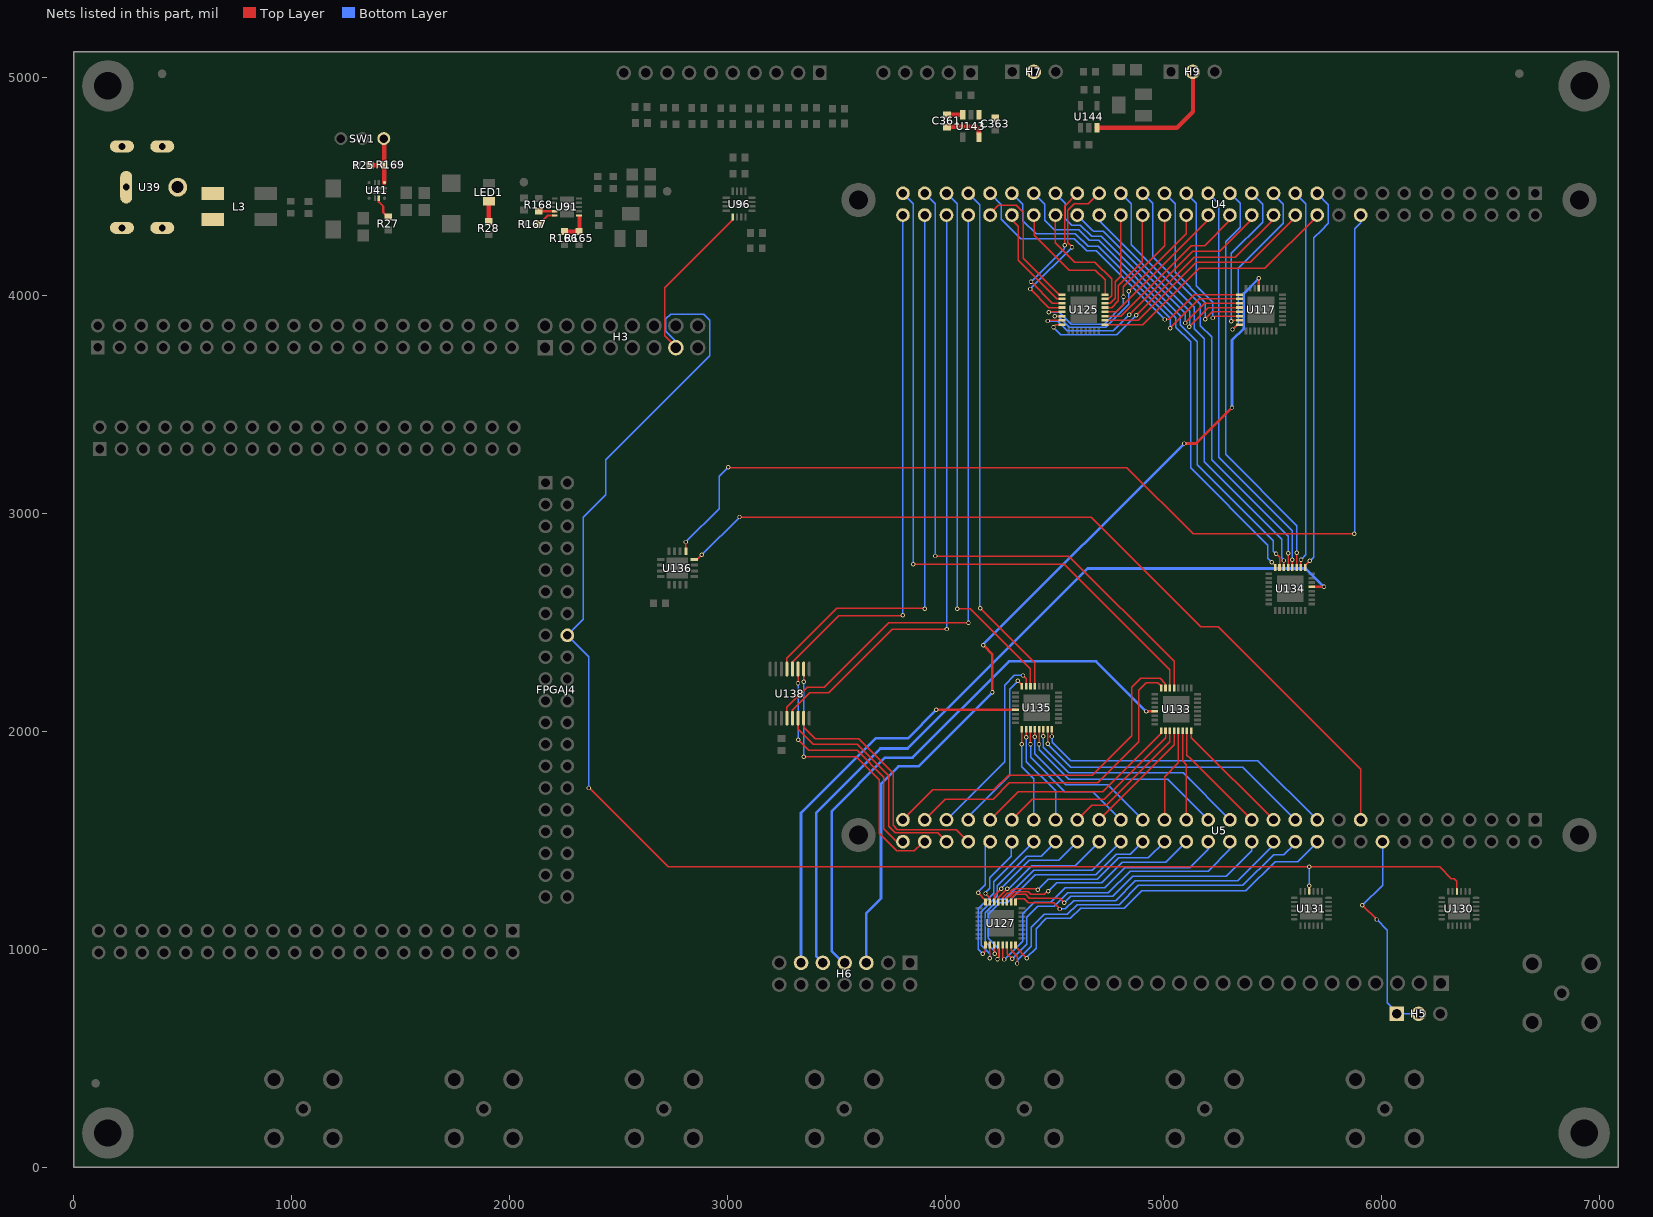
[diagram p0: the nets of this part, all layers, seen from the top]
# Altium PCB MISC82799.PcbDoc (part 4 of 5)
Units mil, origin at the board's own origin, x right, y up, seen from the top; angles counter-clockwise.
Board outline 7086.61 x 5118.11 mil, 4 copper layers (Top Layer, GND, POWER, Bottom Layer); 95 components, 232 nets, 857 pads, 1291 vias.

## Via types
v1: diameter 20, hole 12, Top Layer to Bottom Layer, 1291 vias

## Nets (pads, with @x,y where several pads share a name; then routed paths per layer and width w, separated by ;. In a path a pad name is that pad's centre, name@x,y a point inside that pad or via, vN(x,y) a via of type N, cw(c..) or ccw(c..) an arc to the next point about the centre after c; other vN are vias at no path point) (continued)
NetC361_1: C361.1 U143.3 | length 65.4
  Top Layer w20: C361.1@4006.33,4827.69 U143.3@4071.69,4827.69
NetC361_2: C361.2 U143.5 | length 171.3
  Top Layer w20: C361.2@4006.33,4772.57 4138.43,4772.57 4152,4759 U143.5@4152,4739
NetC363_2: C363.2 H7.2 U143.1
NetH9_2: H9.2 U144.3 | length 654.8
  Top Layer w20: U144.3@4693.96,4767.82 5060.82,4767.82 5135,4842 H9.2@5135,5025
NetL3_1: L3.1 U39.1
NetL3_2: L3.2 U39.2 U39.3
NetLED1_2: LED1.2 R28.2 | length 84.6
  Top Layer w20: R28.2@1905,4347 LED1.2@1905,4431.65
NetR25_2: R25.2 R169.1 SW1.3 U41.1 | length 243.7
  Top Layer w20: R25.2@1360.66,4597 R169.1@1423,4597 ; U41.1@1425.34,4516 R169.1@1425.34,4598 SW1.3@1425.34,4697.34
NetR27_1: R27.1 U41.9 | length 95.3
  Top Layer w10: U41.9@1399.86,4445.37 1399.86,4429.14 1421,4408 1421,4380 R27.1@1436,4365
NetR165_1: R165.1 R166.2 U91.6 | length 137
  Top Layer w20: R166.2@2252,4291.66 2320.66,4291.66 2320.66,4360
NetR167_2: R167.2 U91.5 | length 73.7
  Top Layer w10: R167.2@2146,4336 2175.63,4365.63 U91.5@2207.43,4365.63
NetR168_1: R168.1 U91.4 | length 72.1
  Top Layer w10: R168.1@2135.31,4385.31 U91.4@2207.43,4385.31
PSUB: H5.1 H5.2 U5.16 | length 960.6
  Top Layer w6: v1(5912,1202) v1(5977,1137)
  Bottom Layer w6: v1(5912,1202) 6004.35,1294.35 U5.16@6004.35,1493.8 ; v1(5977,1137) 6026,1088 6026,755 H5.1@6063,718 ; H5.1@6070,704 H5.2@6154,704
S_D_11: U4.26 U125.8 | length 1304.3
  Top Layer w6: v1@4496,3855 4506.1,3865.1 U125.8@4534.58,3865.1 ; v1(4874,3908) 5140,4174 5329,4174 5504.35,4349.35 U4.26@5504.35,4367.81
  Bottom Layer w6: v1(4495,3853) 4529,3819 4785,3819 v1(4874,3908)
S_D_12: U4.28 U125.7 | length 1249.2
  Top Layer w6: v1@4469.78,3884.78 U125.7@4534.58,3884.78 ; v1(4843,3911) 5133,4201 5257,4201 5404.35,4348.35 U4.28@5404.35,4367.81
  Bottom Layer w6: v1(4469,3882) 4515,3882 4559,3838 4770,3838 v1(4843,3911)
S_D_13: U5.28 U127.2 | length 1285.4
  Top Layer w6: U127.2@4301.22,1217.43 4301.22,1233.22 4320,1252 4368,1252 4385,1235 4524,1235 v1(4545,1214)
  Bottom Layer w6: v1@4543,1212 v1(4545,1214) 4575,1244 4767,1244 4859,1336 5288,1336 5404.35,1452.35 U5.28@5404.35,1493.8
S_D_14: U5.26 U127.1 | length 1389.9
  Top Layer w6: U127.1@4320.9,1217.43 4320.9,1225.9 4326,1231 4362,1231 4380,1213 ; 4424,1213 4380,1213 ; v1(4524,1185) 4496,1213 4380,1213
  Bottom Layer w6: v1@4528,1185 4550,1185 4588,1223 4780,1223 4871,1314 5340,1314 U5.26@5504,1478 ; U5.26@5504.35,1478 U5.26@5504.35,1493.8
S_D_21: U4.34 U125.6 | length 946.3
  Top Layer w6: v1(4501,3904) 4502,3905 U125.6@4526,3905 ; v1(4840,4019) 5104.35,4283.35 U4.34@5104.35,4367.81
  Bottom Layer w6: v1(4501,3904) 4517,3904 4567,3854 4734,3854 4840,3960 v1(4840,4019)
S_D_22: U4.36 U125.5 | length 953.5
  Top Layer w6: v1@4473.16,3924.15 U125.5@4534.58,3924.15 ; v1(4816,3993) 4816,4039 5004.35,4227.35 U4.36@5004.35,4367.81
  Bottom Layer w6: v1(4473,3923) 4522,3923 4577,3868 4728,3868 4816,3956 v1(4816,3993)
S_D_23: U5.36 U127.4 | length 892.5
  Top Layer w6: U127.4@4261.84,1217.43 4261.84,1229 U127.4@4261.84,1232.85 ; U127.4@4262,1229 4262,1236 4283.97,1257.97 4292,1257.97 ; 4292.06,1258 4304.53,1270.47 ; 4307.53,1273.47 4304.53,1270.47 ; 4380,1278 4363,1278 ; v1@4419,1274 4415,1278 4363,1278 ; 4304.53,1270.47 4312.06,1278 4363,1278
  Bottom Layer w6: v1(4423,1273) 4472,1322 4696,1322 4794,1420 4930.55,1420 U5.36@5004.35,1493.8
S_D_24: U5.34 U127.3 | length 954.2
  Top Layer w6: U127.3@4281.52,1217.43 4281.52,1234.52 4291,1244 4295,1244 4297,1246 4315.03,1264 4321,1264 ; 4320,1264 4321,1264 ; v1@4467,1267 4452,1252 4391,1252 4379,1264 4321,1264
  Bottom Layer w6: v1(4471,1267) 4510,1306 4717,1306 4810,1399 5009.55,1399 U5.34@5104.35,1493.8
S_D_31: U4.41 U125.4 | length 804.5
  Top Layer w6: v1(4388,4029) 4389,4029 4474.16,3943.85 U125.4@4534.58,3943.85 ; v1@4578,4224 4561,4241 4561,4390 4591,4420 4655,4420 U4.41@4696,4461 ; v1(4580,4221) v1@4580,4224 ; U4.41@4696.77,4460.23 U4.41@4704.35,4467.81
  Bottom Layer w6: v1(4388,4029) v1(4580,4221)
S_D_32: U4.43 U125.3 | length 672.3
  Top Layer w6: v1(4392,4062) 4490.48,3963.52 U125.3@4534.58,3963.52 ; v1@4546,4230 4546,4409.46 U4.43@4604.35,4467.81
  Bottom Layer w6: v1(4392,4062) 4544,4214 v1@4544,4226
  other v1: 4546,4229
S_D_33: U5.44 U127.6 | length 508.1
  Top Layer w6: U127.6@4222.48,1217.43 4222.48,1246.48 v1@4252,1276
  Bottom Layer w6: v1@4256,1279 4385,1408 4518.55,1408 U5.44@4604.35,1493.8
  other v1: 4256,1278
S_D_34: U5.42 U127.5 | length 590.9
  Top Layer w6: U127.5@4242.16,1217.43 4242.16,1236.15 4279,1273 4281.03,1275 v1@4283,1275 ; v1(4283,1278) 4283,1277 4285,1275 v1@4284,1274
  Bottom Layer w6: v1@4284,1273 4287,1276 v1@4287,1278 ; v1@4290,1278 4396,1384 4594.55,1384 U5.42@4704.35,1493.8
S_D_41: U4.50 U125.2 | length 472.6
  Top Layer w6: U4.50@4303,4346 4333,4316 4333,4161 4510.78,3983.22 U125.2@4534.58,3983.22
S_D_42: U4.52 U125.1 | length 630.5
  Top Layer w6: U4.52@4210,4381 4241,4412 4324,4412 4356,4380 4356,4169 4522.1,4002.9 U125.1@4534.58,4002.9
S_D_43: U5.52 U127.8 | length 306.2
  Top Layer w6: v1(4150,1259) 4183.1,1225.9 U127.8@4183.1,1217.43
  Bottom Layer w6: v1@4151,1265 4181,1295 4181,1470.45 U5.52@4204.35,1493.8
S_D_44: U5.50 U127.7 | length 311.1
  Top Layer w6: v1(4183,1256) 4202.78,1236.22 U127.7@4202.78,1217.43
  Bottom Layer w6: v1@4182,1259 4202,1279 4202,1328 4301,1427 U5.50@4301,1474
S_D_51: U4.58 U138.13 | length 2578.5
  Top Layer w6: U138.13@3272.21,2285.82 3272.21,2334.21 3502,2564 v1@3901,2564
  Bottom Layer w6: v1(3904.35,2561.65) U4.58@3904.35,4367.81
S_D_52: U4.60 U138.12 | length 2460.9
  Top Layer w6: U138.12@3297.8,2285.82 3297.8,2315.8 3511,2529 v1@3805,2529
  Bottom Layer w6: v1(3804.35,2532.35) U4.60@3804.35,4367.81
S_D_53: U5.60 U138.11 | length 1152.7
  Top Layer w6: v1@3323.39,2227.61 U138.11@3323.39,2285.82 ; v1(3324,1961) 3373,1912 3594,1912 3717,1789 3717,1764 ; 3717,1787 3717,1764 ; U5.60@3804.35,1493.8 3777.2,1493.8 3717,1554 3717,1764
  Bottom Layer w6: v1(3323,2220) 3324,2220 v1(3324,1961)
S_D_54: U5.58 U138.10 | length 1321.7
  Top Layer w6: v1(3349,1883) 3590,1883 3695,1778 3695,1724 ; v1(3349,2227) U138.10@3349,2262 ; 3695,1773 3695,1724 ; U5.58@3890,1485 3857,1452 3775,1452 3695,1532 3695,1724 ; U5.58@3892.78,1482.22 U5.58@3904.35,1493.8
  Bottom Layer w6: v1(3349,1883) v1(3349,2227)
S_G_11: U4.22 U125.17 | length 1172.9
  Top Layer w6: U125.17@4731.42,3865.1 4905.1,3865.1 5164,4124 5465,4124 5697,4356 U4.22@5697,4360
S_G_12: U4.24 U125.18 | length 1069.3
  Top Layer w6: U125.18@4731.42,3884.78 4884.78,3884.78 5151,4151 5397,4151 5601,4355 U4.24@5601,4360
S_G_13: U5.24 U127.23 | length 1666.2
  Top Layer w6: U127.23@4301.22,1020.57 4301.22,994.78 4328,968 v1(4328,935)
  Bottom Layer w6: v1@4330,936 4330,952 4392,1014 4392,1101 4452,1161 4559,1161 4603,1205 4797,1205 4885,1293 5364,1293 5505,1434 5552,1434 U5.24@5603,1485 ; U5.24@5604.35,1485 U5.24@5604.35,1493.8
S_G_14: U5.22 U127.24 | length 1687.5
  Top Layer w6: U127.24@4320.9,1020.57 4320.9,1011.1 v1(4373,959)
  Bottom Layer w6: v1@4373,963 4416,1006 4416,1095 4463,1142 4573,1142 4619,1188 4819,1188 4899,1268 5378,1268 5512,1402 5616,1402 U5.22@5694,1480 ; U5.22@5692.28,1481.72 U5.22@5704.35,1493.8
S_G_21: U4.30 U125.19 | length 773.4
  Top Layer w6: U125.19@4737,3905 4804,3905 5127,4228 5189,4228 5304.35,4343.35 U4.30@5304.35,4367.81
S_G_22: U4.32 U125.20 | length 660
  Top Layer w6: U125.20@4731.42,3924.15 4782.16,3924.15 U4.32@5213,4355
S_G_23: U5.32 U127.21 | length 1318.7
  Top Layer w6: U127.21@4261.84,1020.57 4261.84,961.15 v1@4266,957
  Bottom Layer w6: v1(4269,953) 4353,1037 4353,1163 4407,1217 4483,1217 4548,1282 4730,1282 4822,1374 5119.35,1374 5204,1458.65 U5.32@5204,1479 ; U5.32@5204.35,1479 U5.32@5204.35,1493.8
S_G_24: U5.30 U127.22 | length 1388.5
  Top Layer w6: U127.22@4282,1013 4282,980 v1(4306,956)
  Bottom Layer w6: v1(4306,956) 4373,1023 4373,1148 4423,1198 4499,1198 4560,1259 4635,1259 ; 4628,1259 4635,1259 ; U5.30@5304.35,1493.8 5304.35,1459.35 5204,1359 4847,1359 4747,1259 4635,1259
S_G_31: U4.38 U125.21 | length 496.6
  Top Layer w6: U125.21@4731.42,3943.85 4762.84,3943.85 4793,3974 4793,4044 4903,4154 U4.38@4903,4351
S_G_32: U4.40 U125.22 | length 427.7
  Top Layer w6: U125.22@4731.42,3963.52 4755.52,3963.52 4778,3986 4778,4061 4804,4087 U4.40@4804,4347
S_G_33: U5.40 U127.19 | length 1001
  Top Layer w6: v1@4222.48,984.52 U127.19@4222.48,1020.57
  Bottom Layer w6: v1(4225,979) 4225,991 4181,1035 4181,1167 4244,1230 4252,1230 4256,1230 4272,1230 4404,1362 4672.55,1362 U5.40@4804.35,1493.8
S_G_34: U5.38 U127.20 | length 1132.6
  Top Layer w6: v1@4240,958 4245,963 4245,991 4242.16,993.85 U127.20@4242.16,1020.57
  Bottom Layer w6: 4246,962 4246,1000 4195,1051 4195,1148 4195,1151 4195,1160 4248,1213 4282,1213 4412,1343 4689,1343 4782,1436 4846.55,1436 U5.38@4904.35,1493.8
  other v1: 4238,954
S_G_41: U4.46 U125.23 | length 566
  Top Layer w6: U4.46@4504,4366 4504,4240 4592,4152 4685,4152 4762,4075 4762,3998 4747.22,3983.22 U125.23@4731.42,3983.22
S_G_42: U4.48 U125.24 | length 560.2
  Top Layer w6: U4.48@4407,4354 4407,4276 4567,4116 4686,4116 4731.42,4070.58 U125.24@4731.42,4002.9 ; U4.48@4408,4354 U4.48@4408,4359
S_G_43: U5.48 U127.17 | length 673.9
  Top Layer w6: v1(4171,979) 4183.1,991.1 U127.17@4183.1,1020.57
  Bottom Layer w6: v1@4170,980 4150,1000 4150,1187 4221,1258 4221,1310 U5.48@4389,1478 ; U5.48@4388.78,1478.22 U5.48@4404.35,1493.8
S_G_44: U5.46 U127.18 | length 792.2
  Top Layer w6: v1(4202.78,959.78) U127.18@4202.78,1020.57
  Bottom Layer w6: v1(4202.78,959.78) 4202.78,979.22 4164,1018 4164,1173 4237,1246 4237,1292 4373,1428 4438.55,1428 U5.46@4504.35,1493.8 ; v1@4203,961 v1@4203,963
S_G_51: U4.54 U138.4 | length 2925.7
  Top Layer w6: U138.4@3272.21,2060.18 3272.21,2109.21 3365,2202 3444,2202 3740,2498 v1(4105,2498)
  Bottom Layer w6: v1@4104.35,2498.35 4104.35,2816 ; 4104.35,2802.65 4104.35,2816 ; U4.54@4104.35,4367.81 4104.35,2816
S_G_52: U4.56 U138.5 | length 2809.8
  Top Layer w6: U138.5@3297.8,2060.18 3297.8,2096.8 3378,2177 3464,2177 3756,2469 v1(4005,2469)
  Bottom Layer w6: v1@4004.35,2469.35 4004.35,2788 ; 4004.35,2774.65 4004.35,2788 ; U4.56@4004.35,4367.81 4004.35,2788
S_G_53: U5.56 U138.6 | length 1081.1
  Top Layer w6: U138.6@3323.39,2060.18 3323.39,2009.61 3393,1940 3595,1940 3739,1796 3739,1564 3768.71,1534.29 3963.85,1534.29 U5.56@4004.35,1493.8
S_G_54: U5.54 U138.7 | length 1154.7
  Top Layer w6: U138.7@3348.98,2060.18 3348.98,2019.02 3402,1966 3601,1966 3759,1808 3759,1568 3779,1548 4050.14,1548 U5.54@4104.35,1493.8
S_N_LEFT: U4.18 U136.9 | length 4937
  Top Layer w6: U136.9@2808.39,2825.77 v1(2808.39,2868.39) ; v1@3004,3214 3008,3210 4832,3210 5135,2907 v1(5875,2907)
  Bottom Layer w6: v1(2808.39,2868.39) 2961,3021 2961,3169 v1(3003,3211) ; v1(5875,2907) 5876,2908 5876,4305 5904.35,4333.35 U4.18@5904.35,4367.81
S_N_RIGHT: U5.17 U136.8 | length 3852.7
  Top Layer w6: U136.8@2846.77,2787.39 2859.39,2787.39 v1(2882,2810) ; v1@3053,2985 v1(3055,2983) 3056,2982 4669,2982 5171,2480 5250,2480 5904.35,1825.65 U5.17@5904.35,1593.8
  Bottom Layer w6: v1(2882,2810) v1(3055,2983)
S_S_11: U4.25 U117.8 | length 757.9
  Top Layer w6: v1(5316,3843) 5338.1,3865.1 U117.8@5348.58,3865.1
  Bottom Layer w6: v1(5316,3843) 5342,3869 5342,4123 5550,4331 5550,4406 5550,4417 U4.25@5518,4449
S_S_12: U4.27 U117.7 | length 698.4
  Top Layer w6: v1@5316.78,3884.78 U117.7@5348.58,3884.78
  Bottom Layer w6: v1(5311,3881) 5311,4193 5454,4336 5454,4418.16 U4.27@5404.35,4467.81
S_S_13: U5.27 U133.7 | length 531.9
  Top Layer w6: U133.7@5107,1997 5107,1891.14 5121.57,1876.57 U5.27@5404.35,1593.8 ; U133.7@5107.22,1997 U133.7@5107.22,2002.57
S_S_14: U5.25 U133.8 | length 565.2
  Top Layer w6: U133.8@5126.9,2002.57 5126.9,1971.1 5138,1960 ; 5138.07,1960.07 U5.25@5504.35,1593.8
S_S_21: U4.33 U117.6 | length 743.3
  Top Layer w6: v1(5225,3896) v1@5229,3896 ; v1@5228,3895 v1@5229,3896 ; U117.6@5348.58,3904.48 5237.48,3904.48 v1@5229,3896
  Bottom Layer w6: U4.33@5104.35,4467.81 5150,4422.16 5150,4043 5225,3968 v1@5225,3903
S_S_22: U4.35 U117.5 | length 821.4
  Top Layer w6: v1(5192,3890) 5192,3892 5224.16,3924.15 U117.5@5348.58,3924.15
  Bottom Layer w6: U4.35@5004.35,4467.81 5053,4419.16 5053,4105 5192,3966 v1@5192,3896
S_S_23: U5.35 U133.5 | length 429.6
  Top Layer w6: U5.35@5004.35,1593.8 5004.35,1791.35 5068,1855 U133.5@5068,1997
S_S_24: U5.33 U133.6 | length 415.7
  Top Layer w6: U133.6@5087.52,2002.57 5087.52,1864.48 5104.35,1847.65 U5.33@5104.35,1593.8
S_S_31: U4.42 U117.4 | length 962.7
  Top Layer w6: v1@5116,3854 5205.84,3943.85 U117.4@5348.58,3943.85
  Bottom Layer w6: U4.42@4704.35,4367.81 4704.35,4342.65 5121,3926 5121,3858 v1(5118,3855) ; v1@5115,3852 v1(5118,3855) ; v1@5118,3853 v1(5118,3855)
S_S_32: U4.44 U117.3 | length 1013.9
  Top Layer w6: v1@5098,3873 5099,3873 5189.52,3963.52 U117.3@5348.58,3963.52
  Bottom Layer w6: U4.44@4604.35,4367.81 4673.08,4299.08 ; 4673,4299 4679,4293 4724,4293 5099,3918 v1(5099,3873.16)
S_S_33: U5.43 U133.3 | length 622.6
  Top Layer w6: U5.43@4604.35,1593.8 4670.55,1660 4737,1660 5028,1951 U133.3@5028,2002
S_S_34: U5.41 U133.4 | length 550.6
  Top Layer w6: U5.41@4704.35,1593.8 5048,1937.45 U133.4@5048,2002
S_S_41: U4.49 U117.2 | length 1433.9
  Top Layer w6: v1@5024,3848 5028,3848 5163.22,3983.22 U117.2@5348.58,3983.22
  Bottom Layer w6: U4.49@4304.35,4467.81 4355,4417.16 4355,4343 4415,4283 4596,4283 4655,4224 4701,4224 5030,3895 v1(5030,3848)
S_S_42: U4.51 U117.1 | length 1465.5
  Top Layer w6: v1@5011,3889 5027,3889 5140.9,4002.9 U117.1@5348.58,4002.9
  Bottom Layer w6: U4.51@4204.35,4467.81 4256,4416.16 4256,4349 4345,4260 4591,4260 4647,4204 4691,4204 v1(5006,3889)
S_S_43: U5.51 U133.1 | length 953.6
  Top Layer w6: U5.51@4204.35,1593.8 4333.55,1723 4720,1723 4989,1992 U133.1@4989,1996
S_S_44: U5.49 U133.2 | length 891.5
  Top Layer w6: U5.49@4304.35,1593.8 4398.55,1688 4727,1688 5009,1970 U133.2@5009,2001
S_S_51: U4.57 U133.21 | length 3104.1
  Top Layer w6: v1(3953,2804) 4566,2804 5048.16,2321.85 U133.21@5048.16,2199.43
  Bottom Layer w6: U4.57@3904.35,4467.81 3953,4419.16 v1(3953,2804) v1@3955,2802
S_S_52: U4.59 U133.22 | length 3177.8
  Top Layer w6: v1(3852,2766) 4544,2766 5028.48,2281.52 U133.22@5028.48,2199.43
  Bottom Layer w6: U4.59@3804.35,4467.81 3852,4420.16 v1@3852,2769
S_S_53: U5.59 U133.23 | length 1627.2
  Top Layer w6: U5.59@3809,1600 3941,1732 4222,1732 4289,1799 4674,1799 4855,1980 4855,2203 4896,2244 4984,2244 5008.78,2219.22 U133.23@5008.78,2199.43
S_S_54: U5.57 U133.24 | length 1485.7
  Top Layer w6: U5.57@3904.35,1593.8 3999.55,1689 4219,1689 4293,1763 4699,1763 4887,1951 4887,2188 4921,2222 4974,2222 U133.24@4986,2210
S_W_11: U4.21 U134.1 | length 1784.9
  Top Layer w6: U134.1@5649.9,2751.43 5649.9,2761.9 v1(5670,2782)
  Bottom Layer w6: v1@5672,2782 5689,2799 5689,3031 ; 5689,3027 5689,3031 ; U4.21@5704.35,4467.81 5756,4416.16 5756,4330 5723,4297 5689,4263 5689,3031
S_W_12: U4.23 U134.2 | length 1744.4
  Top Layer w6: U134.2@5630.22,2751.43 v1(5630.22,2786.78)
  Bottom Layer w6: U4.23@5604.35,4467.81 5653,4419.16 5653,2810 v1@5631,2788
S_W_13: U5.23 U135.7 | length 1342.7
  Top Layer w6: v1(4468.22,1942.22) U135.7@4468.22,2009.57
  Bottom Layer w6: v1@4472,1939 4575,1836 5362.14,1836 U5.23@5604.35,1593.8
S_W_14: U5.21 U135.8 | length 1419.4
  Top Layer w6: v1(4487.9,1976.1) U135.8@4487.9,2009.57
  Bottom Layer w6: v1@4489,1973 4489,1950 4574,1865 4616,1865 5433.14,1865 U5.21@5704.35,1593.8
S_W_21: U4.29 U134.3 | length 1894
  Top Layer w6: U134.3@5610.52,2751.43 v1(5610.52,2818.52)
  Bottom Layer w6: U4.29@5304.35,4467.81 5351,4421.16 5351,4312 5285,4246 5285,3271 5612,2944 v1@5612,2823
S_W_22: U4.31 U134.4 | length 1872.4
  Top Layer w6: U134.4@5590.84,2751.43 v1(5590.84,2786.85)
  Bottom Layer w6: U4.31@5204.35,4467.81 5253,4419.16 5253,3257 5591,2919 v1@5591,2791
S_W_23: U5.31 U135.5 | length 1001.8
  Top Layer w6: v1(4428.84,1940.15) U135.5@4428.84,2009.57
  Bottom Layer w6: v1@4429,1939 4429,1915 4564,1780 5018.14,1780 U5.31@5204.35,1593.8
S_W_24: U5.29 U135.6 | length 1080.5
  Top Layer w6: v1(4448.52,1977.52) U135.6@4448.52,2009.57
  Bottom Layer w6: 4449,1958.52 4449,1952 ; v1@4449,1975 4449,1952 ; U5.29@5304.35,1593.8 5089.14,1809 4566,1809 4449,1926 4449,1952
S_W_31: U4.37 U134.5 | length 1986.8
  Top Layer w6: U134.5@5571.16,2751.43 v1(5571.16,2816.85)
  Bottom Layer w6: U4.37@4904.35,4467.81 4950,4422.16 4950,4177 5169,3958 5169,3860 5220,3809 5220,3246 5572,2894 v1@5572,2823
S_W_32: U4.39 U134.6 | length 2024.5
  Top Layer w6: U134.6@5551.48,2751.43 v1(5551.48,2783.48)
  Bottom Layer w6: U4.39@4804.35,4467.81 4852,4420.16 4852,4232 5140,3944 5140,3847 5186,3801 5186,3237 5542,2881 5542,2795 v1@5552,2785
S_W_33: U5.39 U135.3 | length 667.5
  Top Layer w6: v1(4389.48,1940.52) U135.3@4389.48,2009.57
  Bottom Layer w6: 4390,1921.52 4390,1916 ; v1@4390,1940 4390,1916 ; U5.39@4804.35,1593.8 4675.14,1723 4547,1723 4390,1880 4390,1916
S_W_34: U5.37 U135.4 | length 741.9
  Top Layer w6: v1(4409.16,1975.15) U135.4@4409.16,2009.57
  Bottom Layer w6: 4409,1955 4409,1941 ; v1@4409,1969 4409,1941 ; U5.37@4904.35,1593.8 4744.14,1754 4551,1754 4409,1896 4409,1941
S_W_41: U4.45 U134.7 | length 2196.2
  Top Layer w6: v1(5516,2814) 5531.78,2798.22 U134.7@5531.78,2751.43
  Bottom Layer w6: U4.45@4504.35,4467.81 4550,4422.16 4550,4350 4578,4322 4618,4322 4670,4270 4713,4270 5076,3907 5076,3864 5154,3786 5154,3223 5495.5,2881.5 ; 5499.5,2877.5 5495.5,2881.5 ; v1(5516,2814) 5503,2827 5503,2874 5495.5,2881.5
S_W_42: U4.47 U134.8 | length 2266
  Top Layer w6: v1(5496,2776) 5512.1,2759.9 U134.8@5512.1,2751.43
  Bottom Layer w6: U4.47@4404.35,4467.81 4454,4418.16 4454,4345 4499,4300 4611,4300 4659,4252 4702,4252 5057,3897 5057,3854 5124,3787 5124,3208 5478,2854 5478,2794 v1(5496,2776)
S_W_43: U5.47 U135.1 | length 436.2
  Top Layer w6: v1(4350.1,1940.1) U135.1@4350.1,2009.57
  Bottom Layer w6: v1@4350,1938 4350,1837 4404.35,1782.65 U5.47@4404.35,1593.8
S_W_44: U5.45 U135.2 | length 473.4
  Top Layer w6: v1(4369.78,1972.78) U135.2@4369.78,2009.57
  Bottom Layer w6: 4370,1953.78 4370,1947 ; v1@4370,1968 4370,1947 ; U5.45@4504.35,1593.8 4504.35,1726.65 4370,1861 4370,1947
S_W_51: U4.53 U135.21 | length 2383.8
  Top Layer w6: v1(4159,2564) 4409.16,2313.85 U135.21@4409.16,2206.43
  Bottom Layer w6: U4.53@4104.35,4467.81 4157,4415.16 v1@4157,2567
S_W_52: U4.55 U135.22 | length 2458.6
  Top Layer w6: v1(4053,2562) 4114,2562 4389.48,2286.52 U135.22@4389.48,2206.43
  Bottom Layer w6: U4.55@4004.35,4467.81 4053,4419.16 4053,2799 ; v1@4053,2564 4053,2799 ; 4053,2795 4053,2799
S_W_53: U5.55 U135.23 | length 886
  Top Layer w6: v1(4355,2256) 4369.78,2241.22 U135.23@4369.78,2206.43
  Bottom Layer w6: U5.55@4004.35,1593.8 4271,1860.45 4271,2211 4316,2256 v1(4355,2256)
S_W_54: U5.53 U135.24 | length 762.6
  Top Layer w6: v1(4331,2232) 4350.1,2212.9 U135.24@4350.1,2206.43
  Bottom Layer w6: U5.53@4104.35,1593.8 4104.35,1608.35 4294,1798 4294,2192 v1@4331,2229
SCLK: FPGAJ4.16 H3.13 U96.13 U130.22 U131.22 | length 7907.7
  Top Layer w6: v1@2365,1740 2727,1378 5269,1378 ; H3.13@2756,3770 2712,3814 2712,4034 3023.48,4345.48 U96.13@3023.48,4358.94 ; 5246,1378 5269,1378 ; v1@5664,1378 v1@5668.2,1378 ; U131.22@5668.2,1265.74 v1(5668.2,1291.8) ; U130.22@6345.2,1265.74 6345.2,1289 ; 6345.2,1292 6345.2,1289 ; 5269,1378 v1@5668.2,1378 ; v1@5668.2,1378 6266,1378 6320,1324 6333,1324 6345.2,1311.8 6345.2,1289
  Bottom Layer w6: 2328,2503 2325,2500 ; v1(2363,1740) 2363,2342 FPGAJ4.16@2265,2440 2325,2500 ; H3.13@2760,3771 2760,3792 2717,3835 2717,3892 2739,3914 2891,3914 2919,3886 2919,3723 2442,3246 2442,3085 2338,2981 2338,2513 2325,2500 ; H3.13@2763,3740 H3.13@2763,3741 ; v1(5668.2,1291.8) v1(5668.2,1379.2)
SOURCE_LEFT: H6.5 U117.29 | length 4052.5
  Top Layer w12: v1(4173,2395) 4215,2353 v1(4215,2179) ; v1(5095,3320) 5149,3320 v1(5314,3485) ; U117.29@5437.16,4032.42 v1(5437.16,4078.16)
  Bottom Layer w12: H6.5@3637,938 3637,1166 3704,1233 3704,1759 3784,1839 3875,1839 v1(4215,2179) ; v1@4170,2395 v1(5095,3320) ; v1(5314,3485) 5314,3794 5368,3848 5368,4009 v1(5437.16,4078.16)
SOURCE_RIGHT: H6.7 U133.29 | length 2579.3
  Top Layer w12: v1(4920.16,2091.15) U133.29@4959.58,2091.15
  Bottom Layer w12: H6.7@3531,938 3478,991 3478,1634 3723,1879 3849,1879 4291,2321 4690.31,2321 v1(4920.16,2091.15)
WELL_LEFT: H6.9 U134.29 | length 3585.5
  Top Layer w12: U134.29@5679.42,2662.85 v1(5735.84,2662.85)
  Bottom Layer w12: H6.9@3437,938 3407,968 3407,1627 3701,1921 3826,1921 4652,2747 5651.69,2747 v1(5735.84,2662.85)
WELL_RIGHT: H6.11 U135.29 | length 1876
  Top Layer w12: v1(3956.84,2098.15) 4247,2098.15 ; 4238.16,2098.15 4247,2098.15 ; U135.29@4320.58,2098.15 4247,2098.15
  Bottom Layer w12: H6.11@3337,938 3337,1050 3337,1626 3679,1968 3826.69,1968 v1(3956.84,2098.15)